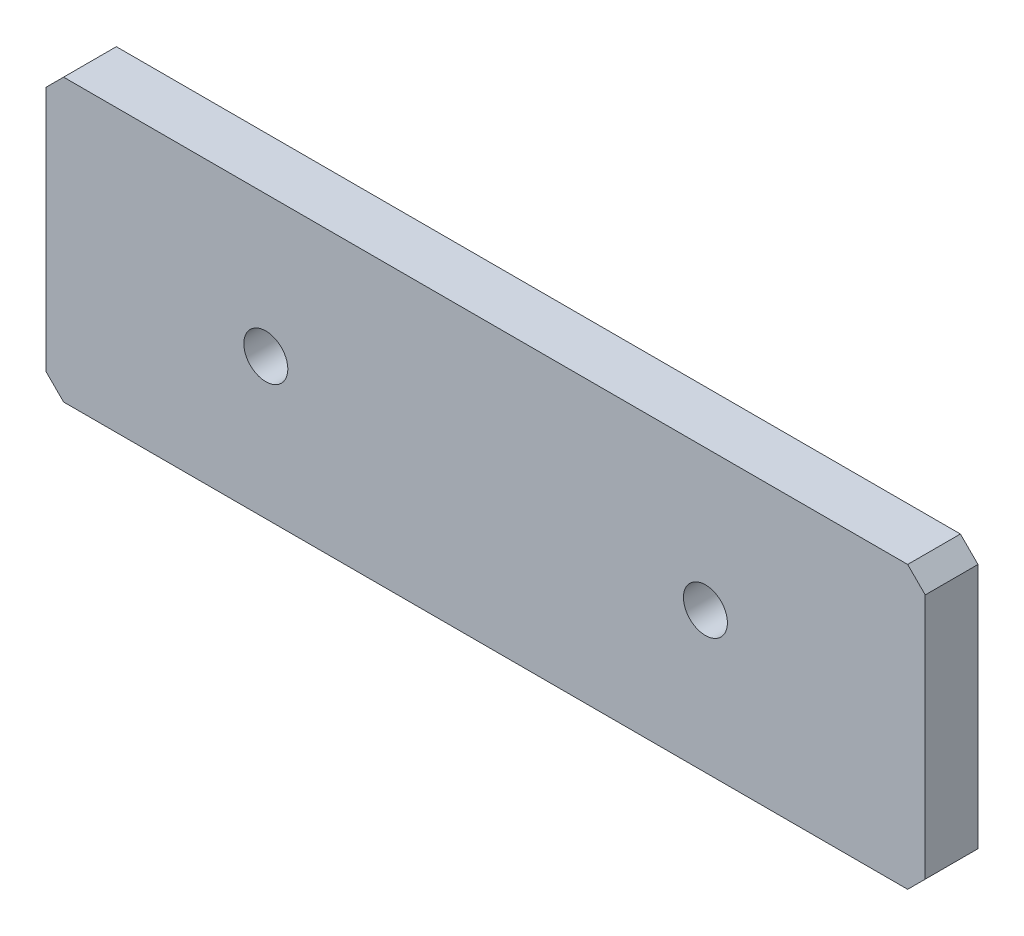
SolidWorks part; units mm, degrees
material "普通碳钢"
ref_plane "前视基准面" through (0, 0, 0) normal (0, 0, 1) x (1, 0, 0)
ref_plane "上视基准面" through (0, 0, 0) normal (0, 1, 0) x (1, 0, 0)
ref_plane "右视基准面" through (0, 0, 0) normal (1, 0, 0) x (0, 0, -1)
sketch "草图1" plane through (0, 0, 0) normal (0, 0, 1) x (1, 0, 0)
  line L1 (-25, 8) -> (25, 8)
  line L2 (-25, 8) -> (-25, -8)
  line L3 (-25, -8) -> (25, -8)
  line L4 (25, 8) -> (25, -8)
  line L5 (-25, 8) -> (25, -8) construction
  line L6 (-25, -8) -> (25, 8) construction
  point P0 (0, 0)
  dimension "D1" = 16
  dimension "D2" = 50
extrude "凸台-拉伸1" add sketch "草图1" along normal mid plane 3
hole_wizard "M3 螺纹孔1" positions "草图3" profile "草图2" tap size "M3" standard "GB" end condition through all
sketch "草图3" plane through (0, 0, -1.5) normal (0, 0, -1) x (-1, 0, 0)
  point P0 (12.5, 0)
  point P2 (-12.5, 0)
  dimension "D1" = 12.5
sketch "草图2" plane through (-12.5, 0, -1.5) normal (1, 0, 0) x (0, 1, 0)
  line L0 (0, 0) -> (0, 3)
  line L1 (0, 3) -> (1.25, 3)
  line L2 (1.25, 3) -> (1.25, 0)
  line L5 (1.25, 0) -> (0, 0)
  line L11 (0, -6.35) -> (0, 107.95) construction
  dimension "通孔螺纹孔钻头直径" = 2.5
  dimension "通孔螺纹孔钻头深度" = 3
cosmetic thread "孔螺蚊线1" parameters "D2"=3
cosmetic thread "孔螺蚊线2" parameters "D2"=3
chamfer "倒角1" distance 1 angle 45 4 edges at (-25, -8, 0) (-25, 8, 0) (25, -8, 0) (25, 8, 0)
